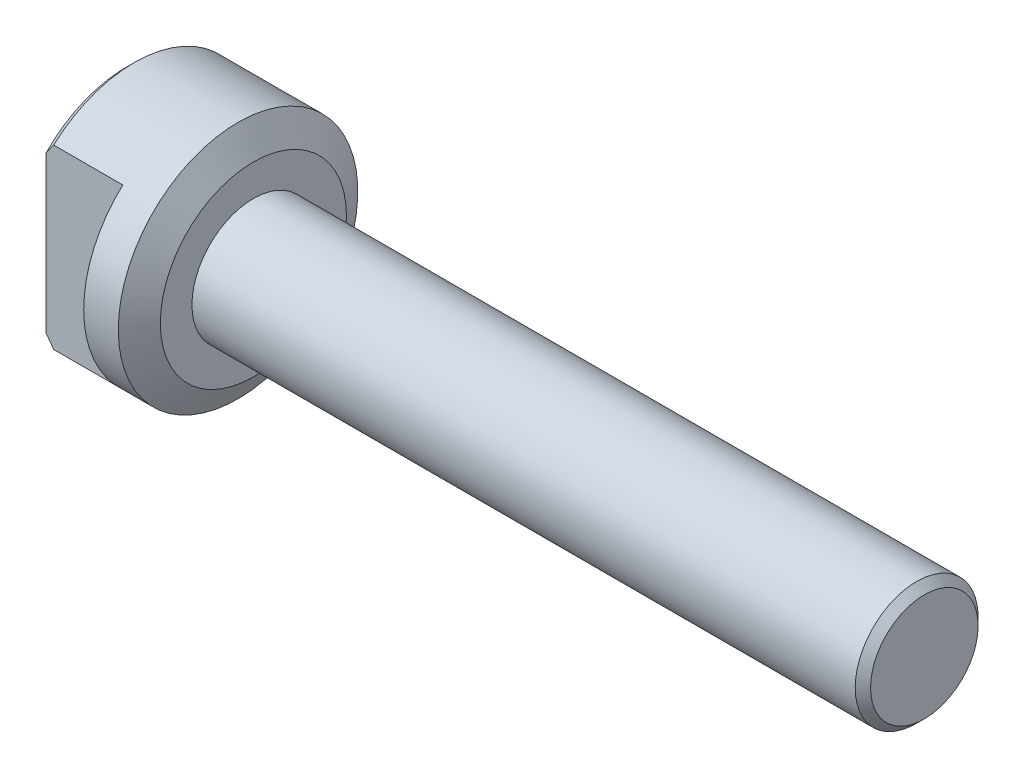
SolidWorks part; units mm, degrees
ref_plane "Front Plane" through (0, 0, 0) normal (0, 0, 1) x (1, 0, 0)
ref_plane "Top Plane" through (0, 0, 0) normal (0, 1, 0) x (1, 0, 0)
ref_plane "Right Plane" through (0, 0, 0) normal (1, 0, 0) x (0, 0, -1)
sketch "Sketch1" plane through (0, 0, 0) normal (0, 0, 1) x (1, 0, 0)
  line L0 (-41.923, 0) -> (58.2098, 0) construction
  line L1 (-26.2107, 0) -> (-26.2107, 15.59)
  line L2 (-26.2107, 15.59) -> (-11.7107, 15.59)
  line L3 (-11.7107, 15.59) -> (-9.7107, 12.12)
  line L4 (-9.7107, 12.12) -> (-9.7107, 8)
  line L5 (-9.7107, 8) -> (77.6393, 8)
  line L6 (77.6393, 8) -> (77.6393, 0)
  line L7 (77.6393, 0) -> (-26.2107, 0)
  dimension "D1" = 15.59
  dimension "D2" = 16.5
  dimension "D3" = 103.85
  dimension "D4" = 14.5
  dimension "D5" = 12.12
  dimension "D6" = 8
revolve "Revolve1" add sketch "Sketch1" angle 360 about L0
chamfer "Chamfer1" distance 1 angle 45 1 edges at (-26.2107, 0, 15.59)
chamfer "Chamfer2" distance 1 angle 45 1 edges at (77.6393, 0, 8)
sketch "Sketch2" plane through (-26.2107, 0, 0) normal (-1, 0, 0) x (0, 0, 1)
  line L1 (-18.7847, 45.255) -> (-10.5, 45.255)
  line L2 (-18.7847, 45.255) -> (-18.7847, -14.745)
  line L3 (-18.7847, -14.745) -> (-10.5, -14.745)
  line L4 (-10.5, 45.255) -> (-10.5, -14.745)
  line L5 (10.5, 15.5606) -> (21.4032, 15.5606)
  line L6 (10.5, 15.5606) -> (10.5, -15.1314)
  line L7 (10.5, -15.1314) -> (21.4032, -15.1314)
  line L8 (21.4032, 15.5606) -> (21.4032, -15.1314)
  dimension "D1" = 10.5
  dimension "D2" = 10.5
  dimension "D3" = 60
extrude "Cut-Extrude1" cut sketch "Sketch2" against normal blind 10
